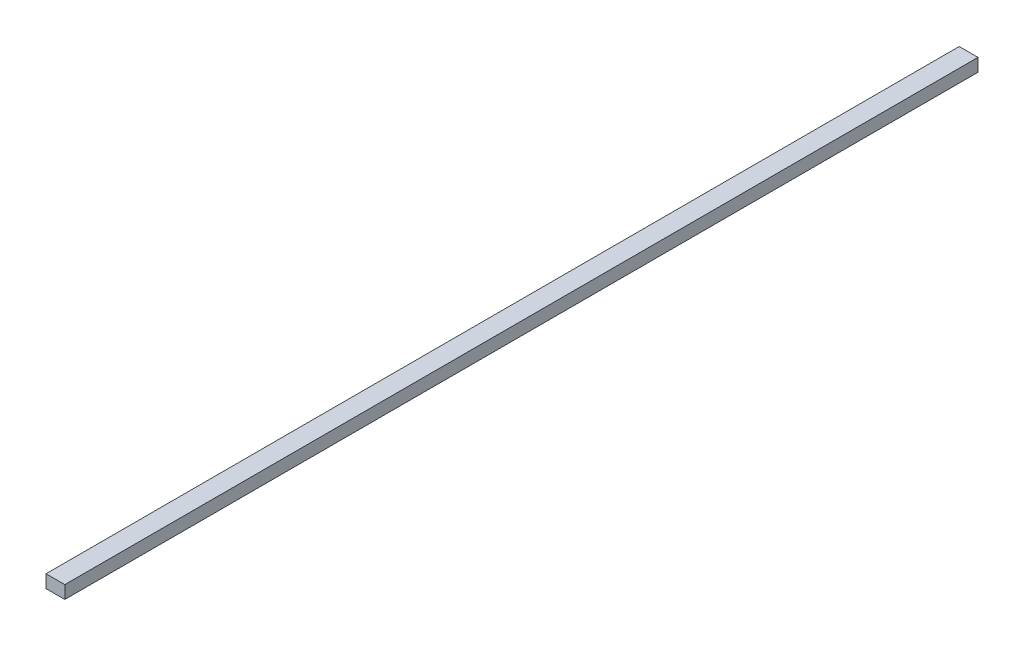
from build123d import *

# Parameters (mm, degrees)
SKETCH1_W           = 7
SKETCH1_H           = 4.8
BOSS_EXTRUDE1_DEPTH = 340


with BuildPart() as part:
    # Sketch1 → Boss-Extrude1 (new body)
    with BuildSketch(Plane.XY):
        with Locations((0, 0.250289017)):
            Rectangle(SKETCH1_W, SKETCH1_H)
    extrude(amount=BOSS_EXTRUDE1_DEPTH)


solid = part.part
